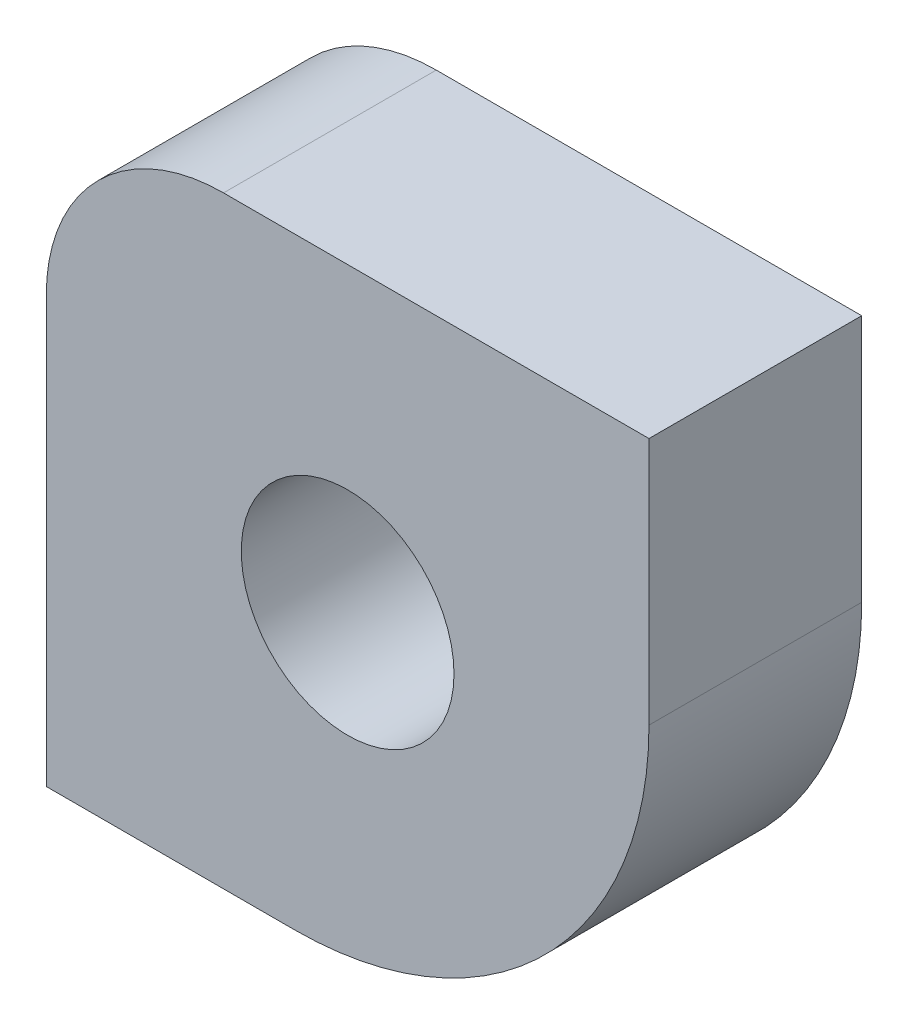
from build123d import *

# Parameters (mm, degrees)
SKETCH1_W           = 17
SKETCH1_H           = 17
BOSS_EXTRUDE1_DEPTH = 6
FILLET1_R           = 10
FILLET2_R           = 5
SKETCH2_R           = 3
CUT_EXTRUDE1_DEPTH  = 6


with BuildPart() as part:
    # Sketch1 → Boss-Extrude1 (new body)
    with BuildSketch(Plane.XY):
        with Locations((8.5, -8.5)):
            Rectangle(SKETCH1_W, SKETCH1_H)
    extrude(amount=BOSS_EXTRUDE1_DEPTH)

    # Fillet1
    fillet1_edges = [part.edges().sort_by_distance(p)[0] for p in [
        (17, -17, 3),
    ]]
    fillet(fillet1_edges, radius=FILLET1_R)

    # Fillet2
    fillet2_edges = [part.edges().sort_by_distance(p)[0] for p in [
        (0, 0, 3),
    ]]
    fillet(fillet2_edges, radius=FILLET2_R)

    # Sketch2 → Cut-Extrude1 (cut)
    with BuildSketch(Plane.XY.offset(6)):
        with Locations((8.5, -8.5)):
            Circle(SKETCH2_R)
    extrude(amount=-CUT_EXTRUDE1_DEPTH, mode=Mode.SUBTRACT)


solid = part.part
